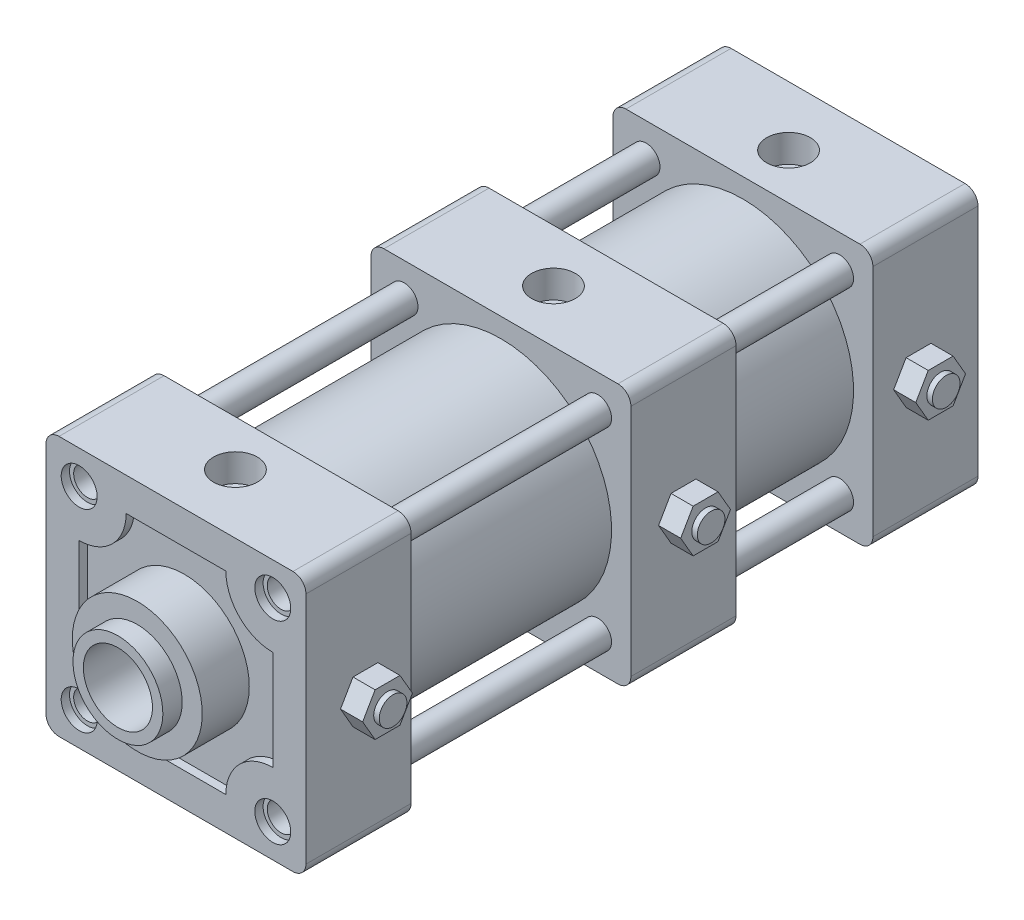
from build123d import *

# Parameters (mm, degrees)
BOSS_EXTRUDE1_DEPTH      = 47
BOSS_EXTRUDE1_DEPTH_BACK = 47
SKETCH4_W                = 38
SKETCH4_H                = 94
BOSS_EXTRUDE2_REACH      = 217.506
SKETCH5_R                = 5
SKETCH6_R                = 5
CUT_EXTRUDE1_DEPTH       = 11
FILLET1_R                = 4.7
SKETCH9_R                = 9
BOSS_EXTRUDE3_DEPTH      = 8
SKETCH10_OUTSIDE_W       = 325.644
SKETCH10_OUTSIDE_H       = 155.644
CUT_EXTRUDE4_DEPTH       = 8
SKETCH11_R               = 5
BOSS_EXTRUDE5_DEPTH      = 2
SKETCH12_R               = 7.903
CUT_EXTRUDE5_DEPTH       = 10
SKETCH8_R                = 12.5
CUT_EXTRUDE6_DEPTH       = 226
CUT_EXTRUDE7_START       = -3
SKETCH13_R               = 6.5
SKETCH13_R_2             = 23.5
CUT_EXTRUDE7_DEPTH       = 3


with BuildPart() as part:
    # Sketch3 → Revolve1 (revolve)
    with BuildSketch(Plane(origin=(0, 0, 0), x_dir=(0, 0, -1), z_dir=(1, 0, 0))):
        Polygon((0, 0), (-264, 0), (-264, 16.25), (-257, 16.25), (-257, 23.5), (-243, 23.5), (-243, 47), (-205, 47), (-205, 40), (-125.5, 40), (-125.5, 47), (-87.5, 47), (-87.5, 40), (-38, 40), (-38, 47), (0, 47), align=None)
    revolve(axis=Axis((0, 0, 0), (0, 0, 1)))

    # Sketch4 → Boss-Extrude1 (add, two sides: drawn at the far end of the back side and taken through both)
    with BuildSketch(Plane(origin=(0, 0, 0), x_dir=(0, 0, -1), z_dir=(1, 0, 0)).offset(-BOSS_EXTRUDE1_DEPTH_BACK)):
        with Locations((-224, 0)):
            Rectangle(SKETCH4_W, SKETCH4_H)
        with Locations((-106.5, 0)):
            Rectangle(SKETCH4_W, SKETCH4_H)
        with Locations((-19, 0)):
            Rectangle(SKETCH4_W, SKETCH4_H)
    extrude(amount=BOSS_EXTRUDE1_DEPTH + BOSS_EXTRUDE1_DEPTH_BACK)

    # Sketch5 → Boss-Extrude2 (add, up to next)
    with BuildSketch(Plane(origin=(0, 0, 205), x_dir=(-1, 0, 0), z_dir=(0, 0, -1)), mode=Mode.PRIVATE) as boss_extrude2_sk1:
        with Locations(Location((-35, 35, 0), (0, 0, 270))):
            Circle(SKETCH5_R)
    boss_extrude2_tool1 = extrude(boss_extrude2_sk1.sketch, amount=BOSS_EXTRUDE2_REACH, mode=Mode.PRIVATE) - part.part
    # Sketch5 → Boss-Extrude2 (add, up to next)
    with BuildSketch(Plane(origin=(0, 0, 205), x_dir=(-1, 0, 0), z_dir=(0, 0, -1)), mode=Mode.PRIVATE) as boss_extrude2_sk2:
        with Locations(Location((35, 35, 0), (0, 0, 270))):
            Circle(SKETCH5_R)
    boss_extrude2_tool2 = extrude(boss_extrude2_sk2.sketch, amount=BOSS_EXTRUDE2_REACH, mode=Mode.PRIVATE) - part.part
    # Sketch5 → Boss-Extrude2 (add, up to next)
    with BuildSketch(Plane(origin=(0, 0, 205), x_dir=(-1, 0, 0), z_dir=(0, 0, -1)), mode=Mode.PRIVATE) as boss_extrude2_sk3:
        with Locations(Location((-35, -35, 0), (0, 0, 270))):
            Circle(SKETCH5_R)
    boss_extrude2_tool3 = extrude(boss_extrude2_sk3.sketch, amount=BOSS_EXTRUDE2_REACH, mode=Mode.PRIVATE) - part.part
    # Sketch5 → Boss-Extrude2 (add, up to next)
    with BuildSketch(Plane(origin=(0, 0, 205), x_dir=(-1, 0, 0), z_dir=(0, 0, -1)), mode=Mode.PRIVATE) as boss_extrude2_sk4:
        with Locations(Location((35, -35, 0), (0, 0, 270))):
            Circle(SKETCH5_R)
    boss_extrude2_tool4 = extrude(boss_extrude2_sk4.sketch, amount=BOSS_EXTRUDE2_REACH, mode=Mode.PRIVATE) - part.part
    add(boss_extrude2_tool1.solids().sort_by_distance((35, 35, 205))[0])
    add(boss_extrude2_tool1.solids().sort_by_distance((35, 35, 205))[1])
    add(boss_extrude2_tool2.solids().sort_by_distance((-35, 35, 205))[0])
    add(boss_extrude2_tool2.solids().sort_by_distance((-35, 35, 205))[1])
    add(boss_extrude2_tool3.solids().sort_by_distance((35, -35, 205))[0])
    add(boss_extrude2_tool3.solids().sort_by_distance((35, -35, 205))[1])
    add(boss_extrude2_tool4.solids().sort_by_distance((-35, -35, 205))[0])
    add(boss_extrude2_tool4.solids().sort_by_distance((-35, -35, 205))[1])

    # Sketch6 → Cut-Extrude1 (cut)
    with BuildSketch(Plane.XY.offset(243)):
        with Locations(Location((-35, 35, 0), (0, 0, 270))):
            Circle(SKETCH6_R)
        with Locations(Location((35, 35, 0), (0, 0, 270))):
            Circle(SKETCH6_R)
        with Locations(Location((-35, -35, 0), (0, 0, 270))):
            Circle(SKETCH6_R)
        with Locations(Location((35, -35, 0), (0, 0, 270))):
            Circle(SKETCH6_R)
    extrude(amount=-CUT_EXTRUDE1_DEPTH, mode=Mode.SUBTRACT)

    # Fillet1
    fillet1_edges = [part.edges().sort_by_distance(p)[0] for p in [
        (-47, -47, 224),
        (47, -47, 224),
        (-47, 47, 224),
        (47, 47, 224),
        (-47, -47, 106.5),
        (47, 47, 106.5),
        (-47, 47, 106.5),
        (47, -47, 106.5),
        (-47, -47, 19),
        (47, 47, 19),
        (-47, 47, 19),
        (47, -47, 19),
    ]]
    fillet(fillet1_edges, radius=FILLET1_R)

    # Sketch9 → Boss-Extrude3 (add)
    with BuildSketch(Plane(origin=(47, 0, 0), x_dir=(0, 0, -1), z_dir=(1, 0, 0))):
        with Locations(Location((-221.5, 0, 0), (0, 0, 180))):
            Circle(SKETCH9_R)
        with Locations((-106.5, 0)):
            Circle(SKETCH9_R)
        with Locations((-21.5, 0)):
            Circle(SKETCH9_R)
    extrude(amount=BOSS_EXTRUDE3_DEPTH)

    # Sketch10 outside → Cut-Extrude4 (cut)
    with BuildSketch(Plane(origin=(55, 0, 0), x_dir=(0, 0, -1), z_dir=(1, 0, 0))):
        with Locations((-132, 0)):
            Rectangle(SKETCH10_OUTSIDE_W, SKETCH10_OUTSIDE_H)
        Polygon((-217, -7.794228634), (-212.5, 0), (-217, 7.794228634), (-226, 7.794228634), (-230.5, 0), (-226, -7.794228634), align=None, mode=Mode.SUBTRACT)
        Polygon((-102, -7.794228634), (-97.5, 0), (-102, 7.794228634), (-111, 7.794228634), (-115.5, 0), (-111, -7.794228634), align=None, mode=Mode.SUBTRACT)
        Polygon((-17, -7.794228634), (-12.5, 0), (-17, 7.794228634), (-26, 7.794228634), (-30.5, 0), (-26, -7.794228634), align=None, mode=Mode.SUBTRACT)
    extrude(amount=-CUT_EXTRUDE4_DEPTH, mode=Mode.SUBTRACT)

    # Sketch11 → Boss-Extrude5 (add)
    with BuildSketch(Plane(origin=(55, 0, 0), x_dir=(0, 0, -1), z_dir=(1, 0, 0))):
        with Locations((-221.5, 0)):
            Circle(SKETCH11_R)
        with Locations((-106.5, 0)):
            Circle(SKETCH11_R)
        with Locations((-21.5, 0)):
            Circle(SKETCH11_R)
    extrude(amount=BOSS_EXTRUDE5_DEPTH)

    # Sketch12 → Cut-Extrude5 (cut)
    with BuildSketch(Plane(origin=(0, 47, 0), x_dir=(1, 0, 0), z_dir=(0, 1, 0))):
        with Locations(Location((0, -221.5, 0), (0, 0, 270))):
            Circle(SKETCH12_R)
        with Locations(Location((0, -106.5, 0), (0, 0, 270))):
            Circle(SKETCH12_R)
        with Locations(Location((0, -21.5, 0), (0, 0, 270))):
            Circle(SKETCH12_R)
    extrude(amount=-CUT_EXTRUDE5_DEPTH, mode=Mode.SUBTRACT)

    # Sketch8 → Cut-Extrude6 (cut)
    with BuildSketch(Plane.XY.offset(264)):
        Circle(SKETCH8_R)
    extrude(amount=-CUT_EXTRUDE6_DEPTH, mode=Mode.SUBTRACT)

    # Sketch13 → Cut-Extrude7 (cut)
    # profile 1 of 5: a face of its own
    with BuildSketch(Plane.XY.offset(243).offset(CUT_EXTRUDE7_START)):
        with Locations((-35, 35)):
            Circle(SKETCH13_R)
    # profile 2 of 5: a face of its own
    with BuildSketch(Plane.XY.offset(243).offset(CUT_EXTRUDE7_START)):
        with Locations((35, 35)):
            Circle(SKETCH13_R)
    # profile 3 of 5: a face of its own
    with BuildSketch(Plane.XY.offset(243).offset(CUT_EXTRUDE7_START)):
        with Locations((35, -35)):
            Circle(SKETCH13_R)
    # profile 4 of 5: a face of its own
    with BuildSketch(Plane.XY.offset(243).offset(CUT_EXTRUDE7_START)):
        with Locations((-35, -35)):
            Circle(SKETCH13_R)
    # profile 5 of 5: a face of its own
    with BuildSketch(Plane.XY.offset(243).offset(CUT_EXTRUDE7_START)):
        with BuildLine():
            Line((-35, -18.029437252), (-35, 18.029437252))
            ThreePointArc((-35, 18.029437252), (-23, 23), (-18.029437252, 35))
            Line((-18.029437252, 35), (18.029437252, 35))
            ThreePointArc((18.029437252, 35), (23, 23), (35, 18.029437252))
            Line((35, 18.029437252), (35, -18.029437252))
            ThreePointArc((35, -18.029437252), (23, -23), (18.029437252, -35))
            Line((18.029437252, -35), (-18.029437252, -35))
            ThreePointArc((-18.029437252, -35), (-23, -23), (-35, -18.029437252))
        make_face()
        with Locations(Location((0, 0, 0), (0, 0, 90))):
            Circle(SKETCH13_R_2, mode=Mode.SUBTRACT)
    extrude(amount=CUT_EXTRUDE7_DEPTH, mode=Mode.SUBTRACT)


solid = part.part
